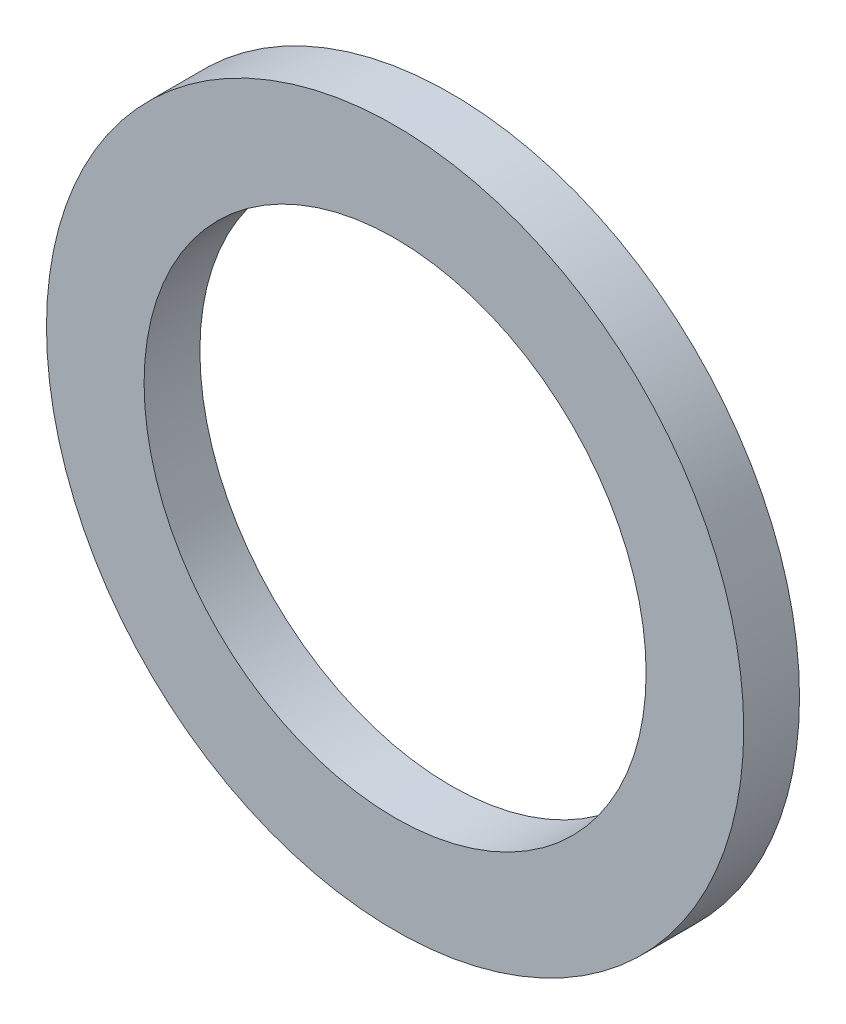
from build123d import *

# Parameters (mm, degrees)
SKETCH_1_R      = 25
SKETCH_1_R_2    = 18
EXTRUDE_1_DEPTH = 4


with BuildPart() as part:
    # 草图1 → 凸台-拉伸1 (new body)
    with BuildSketch(Plane.XY):
        Circle(SKETCH_1_R)
        Circle(SKETCH_1_R_2, mode=Mode.SUBTRACT)
    extrude(amount=EXTRUDE_1_DEPTH)


solid = part.part
